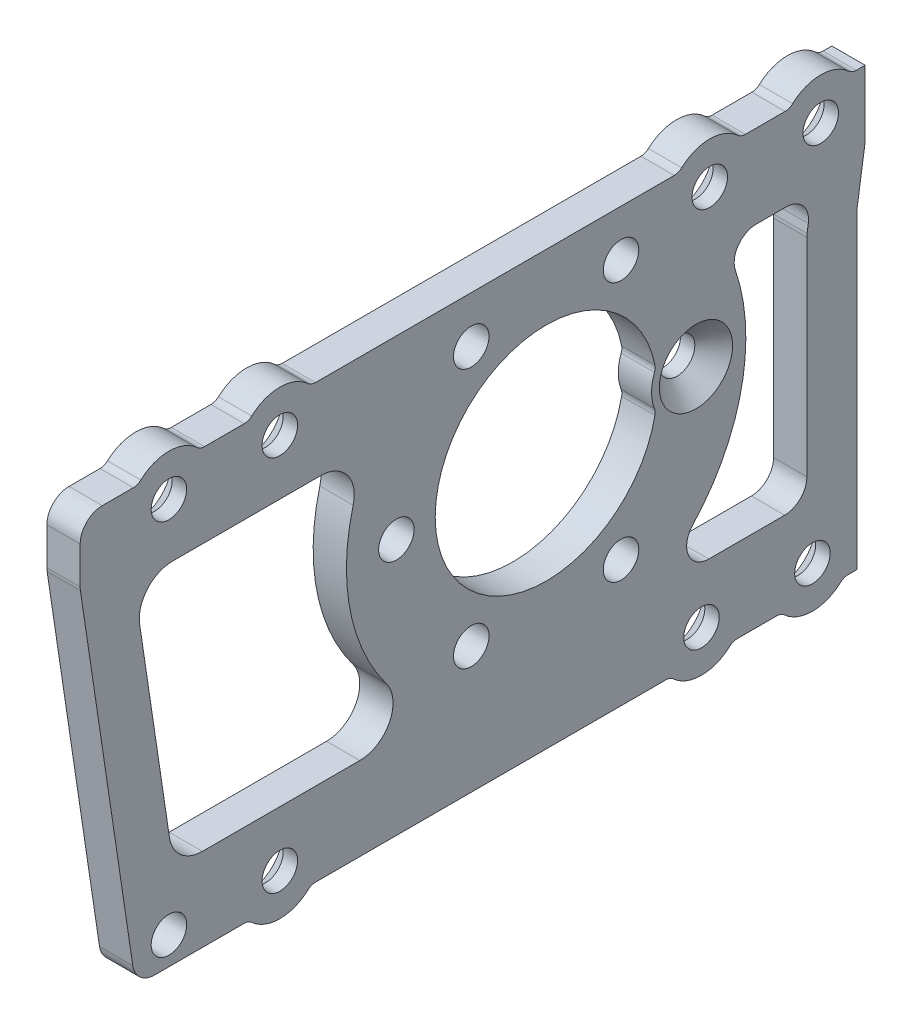
from build123d import *

# Parameters (mm, degrees)
SKETCH_1_R                   = 1.6
SKETCH_1_R_2                 = 10
EXTRUDE_1_DEPTH              = 3
SKETCH_2_R                   = 3.75
SKETCH_2_R_2                 = 1.6
SKETCH_2_R_3                 = 4
EXTRUDE_2_DEPTH              = 3
HOLE_WIZARD_M3_1_D           = 3.2
HOLE_WIZARD_M3_1_DEPTH       = 7.5
HOLE_WIZARD_M3_1_CSINK_D     = 6.6
HOLE_WIZARD_M3_1_CSINK_ANGLE = 90
HOLE_WIZARD_M3_1_TIP         = 0.96137699
CUT_EXTRUDE_1_DEPTH          = 10
HOLE_WIZARD_M3_2_D           = 3.2
HOLE_WIZARD_M3_2_DEPTH       = 7.5
HOLE_WIZARD_M3_2_CSINK_D     = 6.6
HOLE_WIZARD_M3_2_CSINK_ANGLE = 90
HOLE_WIZARD_M3_2_TIP         = 0.96137699
FILLET_1_R                   = 3
FILLET_2_R                   = 2
FILLET_3_R                   = 1


with BuildPart() as part:
    # 草图1 → 凸台-拉伸1 (new body)
    with BuildSketch(Plane(origin=(0, 0, 0), x_dir=(0, 0, -1), z_dir=(1, 0, 0))):
        Polygon((28, 4.9), (28, -23.1), (-37, -23.1), (-42, 10.4), (-42, 15.9), (28.75, 15.9), (28.75, 9.9), align=None)
        with Locations((-13.5, 0)):
            Circle(SKETCH_1_R, mode=Mode.SUBTRACT)
        with Locations((-6.75, 11.691342951)):
            Circle(SKETCH_1_R, mode=Mode.SUBTRACT)
        with Locations((6.75, 11.691342951)):
            Circle(SKETCH_1_R, mode=Mode.SUBTRACT)
        with Locations((13.5, 0)):
            Circle(SKETCH_1_R, mode=Mode.SUBTRACT)
        with Locations((6.75, -11.691342951)):
            Circle(SKETCH_1_R, mode=Mode.SUBTRACT)
        with Locations((-6.75, -11.691342951)):
            Circle(SKETCH_1_R, mode=Mode.SUBTRACT)
        Circle(SKETCH_1_R_2, mode=Mode.SUBTRACT)
        with Locations((14, -20.6)):
            Circle(SKETCH_1_R, mode=Mode.SUBTRACT)
        with Locations((24, -20.6)):
            Circle(SKETCH_1_R, mode=Mode.SUBTRACT)
        with Locations((24.75, 13.4)):
            Circle(SKETCH_1_R, mode=Mode.SUBTRACT)
        with Locations((14.75, 13.4)):
            Circle(SKETCH_1_R, mode=Mode.SUBTRACT)
        with Locations((-24, -20.6)):
            Circle(SKETCH_1_R, mode=Mode.SUBTRACT)
        with Locations((-34, -20.6)):
            Circle(SKETCH_1_R, mode=Mode.SUBTRACT)
        with Locations((-34, 13.4)):
            Circle(SKETCH_1_R, mode=Mode.SUBTRACT)
        with Locations((-24, 13.4)):
            Circle(SKETCH_1_R, mode=Mode.SUBTRACT)
    extrude(amount=EXTRUDE_1_DEPTH)

    # 草图2 → 凸台-拉伸2 (add)
    # profile 1 of 8: a face of its own
    with BuildSketch(Plane.ZY):
        with Locations((-24.75, 13.4)):
            Circle(SKETCH_2_R)
        with Locations(Location((-24.75, 13.4, 0), (0, 0, 180))):
            Circle(SKETCH_2_R_2, mode=Mode.SUBTRACT)
    # profile 2 of 8: a face of its own
    with BuildSketch(Plane.ZY):
        with Locations((-14.75, 13.4)):
            Circle(SKETCH_2_R)
        with Locations(Location((-14.75, 13.4, 0), (0, 0, 180))):
            Circle(SKETCH_2_R_2, mode=Mode.SUBTRACT)
    # profile 3 of 8: a face of its own
    with BuildSketch(Plane.ZY):
        with Locations((24, 13.4)):
            Circle(SKETCH_2_R)
        with Locations(Location((24, 13.4, 0), (0, 0, 180))):
            Circle(SKETCH_2_R_2, mode=Mode.SUBTRACT)
    # profile 4 of 8: a face of its own
    with BuildSketch(Plane.ZY):
        with Locations((24, -20.6)):
            Circle(SKETCH_2_R)
        with Locations(Location((24, -20.6, 0), (0, 0, 180))):
            Circle(SKETCH_2_R_2, mode=Mode.SUBTRACT)
    # profile 5 of 8: a face of its own
    with BuildSketch(Plane.ZY):
        with Locations((-24, -20.6)):
            Circle(SKETCH_2_R)
        with Locations(Location((-24, -20.6, 0), (0, 0, 180))):
            Circle(SKETCH_2_R_2, mode=Mode.SUBTRACT)
    # profile 6 of 8: a face of its own
    with BuildSketch(Plane.ZY):
        with Locations((-14, -20.6)):
            Circle(SKETCH_2_R)
        with Locations(Location((-14, -20.6, 0), (0, 0, 180))):
            Circle(SKETCH_2_R_2, mode=Mode.SUBTRACT)
    # profile 7 of 8: a face of its own
    with BuildSketch(Plane.ZY):
        with Locations((-13.5, 0)):
            Circle(SKETCH_2_R_3)
        with Locations(Location((-13.5, 0, 0), (0, 0, 180))):
            Circle(SKETCH_2_R_2, mode=Mode.SUBTRACT)
    # profile 8 of 8: a face of its own
    with BuildSketch(Plane.ZY):
        with Locations((34, 13.4)):
            Circle(SKETCH_2_R)
        with Locations(Location((34, 13.4, 0), (0, 0, 180))):
            Circle(SKETCH_2_R_2, mode=Mode.SUBTRACT)
    extrude(amount=-EXTRUDE_2_DEPTH)

    # M3 十字槽半沉头木螺钉的锥形沉头孔1
    with Locations(Plane.ZY):
        with Locations((-24.75, 13.4), (-14.75, 13.4), (-24, -20.6), (-14, -20.6), (24, 13.4), (34, 13.4), (24, -20.6)):
            CounterSinkHole(HOLE_WIZARD_M3_1_D / 2, HOLE_WIZARD_M3_1_CSINK_D / 2, depth=HOLE_WIZARD_M3_1_DEPTH, counter_sink_angle=HOLE_WIZARD_M3_1_CSINK_ANGLE)
            with Locations((0, 0, -(HOLE_WIZARD_M3_1_DEPTH + HOLE_WIZARD_M3_1_TIP / 2))):  # 118° drill point
                Cone(0, HOLE_WIZARD_M3_1_D / 2, HOLE_WIZARD_M3_1_TIP, mode=Mode.SUBTRACT)

    # 草图17 → 切除-拉伸1 (cut)
    with BuildSketch(Plane.ZY):
        with BuildLine():
            Line((37.15164609, 8.4), (15.919798994, 8.4))
            ThreePointArc((15.919798994, 8.4), (17.472211965, 4.326870585), (18, 0))
            ThreePointArc((18, 0), (15.582676264, -9.010005574), (8.979977728, -15.6))
            Line((8.979977728, -15.6), (33.569556538, -15.6))
            Line((33.569556538, -15.6), (37.15164609, 8.4))
        make_face()
        with BuildLine():
            ThreePointArc((-8.979977728, -15.6), (-17.291608375, -5.00002798), (-15.919798994, 8.4))
            Line((-15.919798994, 8.4), (-23.974656606, 8.4))
            Line((-23.974656606, 8.4), (-23.5, 5.235622624))
            Line((-23.5, 5.235622624), (-23.5, -15.6))
            Line((-23.5, -15.6), (-8.979977728, -15.6))
        make_face()
    extrude(amount=-CUT_EXTRUDE_1_DEPTH, mode=Mode.SUBTRACT)

    # M3 十字槽半沉头木螺钉的锥形沉头孔2
    with Locations(Plane(origin=(3, 0, 0), x_dir=(0, 0, -1), z_dir=(1, 0, 0))):
        with Locations((13.5, 0)):
            CounterSinkHole(HOLE_WIZARD_M3_2_D / 2, HOLE_WIZARD_M3_2_CSINK_D / 2, depth=HOLE_WIZARD_M3_2_DEPTH, counter_sink_angle=HOLE_WIZARD_M3_2_CSINK_ANGLE)
            with Locations((0, 0, -(HOLE_WIZARD_M3_2_DEPTH + HOLE_WIZARD_M3_2_TIP / 2))):  # 118° drill point
                Cone(0, HOLE_WIZARD_M3_2_D / 2, HOLE_WIZARD_M3_2_TIP, mode=Mode.SUBTRACT)

    # 圆角1
    fillet_1_edges = [part.edges().sort_by_distance(p)[0] for p in [
        (1.5, -15.6, 8.979977728),
        (1.5, 8.4, 15.919798994),
        (1.5, 8.4, 37.15164609),
        (1.5, -15.6, 33.569556538),
    ]]
    fillet(fillet_1_edges, radius=FILLET_1_R)

    # 圆角2
    fillet_2_edges = [part.edges().sort_by_distance(p)[0] for p in [
        (1.5, 9.9, -28.75),
        (1.5, 4.9, -28),
        (1.5, -23.1, 37),
        (1.5, 10.4, 42),
        (1.5, 15.9, 42),
        (1.5, 8.4, -15.919798994),
        (1.5, -15.6, -8.979977728),
        (1.5, -15.6, -23.5),
        (1.5, 5.235622624, -23.5),
        (1.5, 8.4, -23.974656606),
    ]]
    fillet(fillet_2_edges, radius=FILLET_2_R)

    # 圆角3
    fillet_3_edges = [part.edges().sort_by_distance(p)[0] for p in [
        (1.5, 15.9, -11.954915028),
        (1.5, 15.9, -17.545084972),
        (1.5, 15.9, 26.795084972),
        (1.5, 15.9, 21.204915028),
        (1.5, -23.1, 26.795084972),
        (1.5, -23.1, 21.204915028),
        (1.5, -23.1, -26.795084972),
        (1.5, -23.1, -21.204915028),
        (1.5, -23.1, -16.795084972),
        (1.5, -23.1, -11.204915028),
        (1.5, 1.660869548, -9.861111111),
        (1.5, -1.660869548, -9.861111111),
        (1.5, 15.9, 36.795084972),
        (1.5, 15.9, 31.204915028),
        (1.5, 15.9, -27.545084972),
        (1.5, 15.9, -21.954915028),
    ]]
    fillet(fillet_3_edges, radius=FILLET_3_R)


solid = part.part
